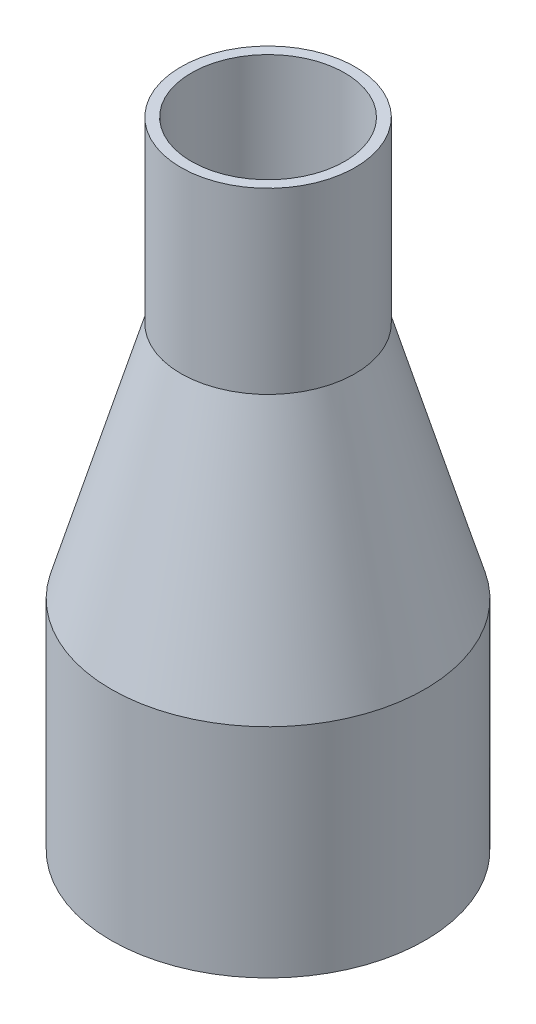
from build123d import *


with BuildPart() as part:
    # Sketch 1 → Revolve 1 (revolve)
    with BuildSketch(Plane.XY, mode=Mode.PRIVATE) as revolve_1_sk:
        Polygon((-12.5, 45.5), (-12.5, 19.9), (-22.5, -14.3), (-22.5, -45.5), (-21, -45.5), (-21, -14.514801212), (-11, 19.685198788), (-11, 45.5), align=None)
    revolve(revolve_1_sk.sketch.rotate(Axis((0, 22.245762712, 0), (0, -1, 0)), 270), axis=Axis((0, 22.245762712, 0), (0, -1, 0)))


solid = part.part
